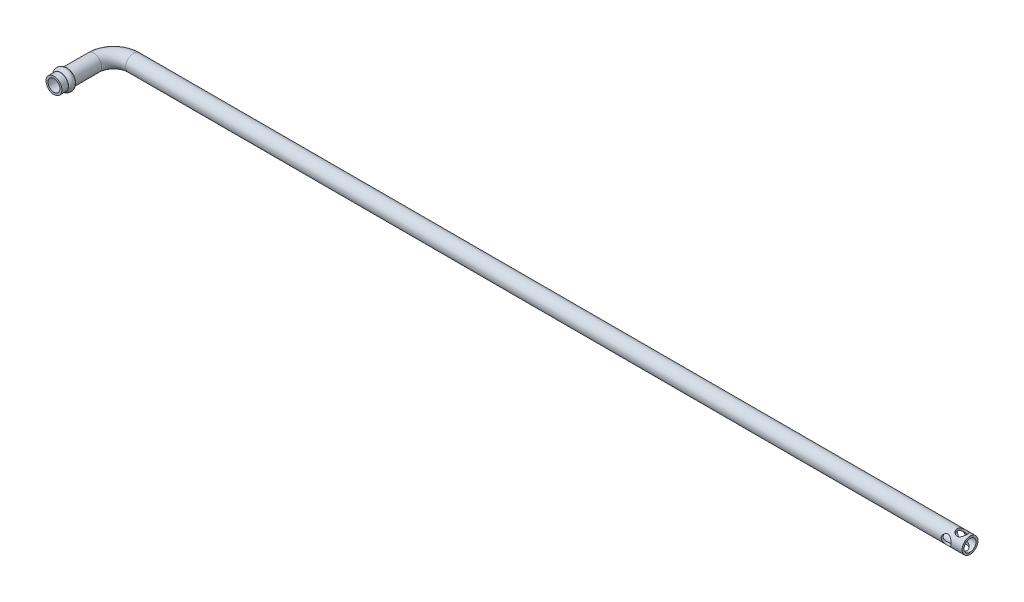
from build123d import *

# Parameters (mm, degrees)
SKETCH1_R               = 4
SKETCH1_R_2             = 3
FILLET1_R               = 0.1
CUT_EXTRUDE1_DEPTH      = 432.371069971
CUT_EXTRUDE1_DEPTH_BACK = 432.371069971
SKETCH4_R               = 2.5
CUT_EXTRUDE2_DEPTH      = 432.371070071
CUT_EXTRUDE2_DEPTH_BACK = 432.371070071
SKETCH5_R               = 2.5


with BuildPart() as part:
    # Sweep1: sweep along a path in Sketch2
    with BuildLine(Plane(origin=(0, 0, 0), x_dir=(1, 0, 0), z_dir=(0, 1, 0))) as sweep1_path:
        Line((0, 0), (0, 20))
        ThreePointArc((0, 20), (2.928932188, 27.071067812), (10, 30))
        Line((10, 30), (430, 30))
    # Sketch1 → Sweep1 (sweep)
    with BuildSketch(Plane.XY):
        Circle(SKETCH1_R)
        Circle(SKETCH1_R_2, mode=Mode.SUBTRACT)
    sweep(path=sweep1_path.line)

    # Sketch3 → Revolve1 (revolve)
    with BuildSketch(Plane(origin=(0, 0, 0), x_dir=(1, 0, 0), z_dir=(0, 1, 0)), mode=Mode.PRIVATE) as revolve1_sk:
        with BuildLine():
            Line((-4, 6.732050808), (-4, 3.267949192))
            ThreePointArc((-4, 3.267949192), (-5, 5), (-4, 6.732050808))
        make_face()
    revolve(revolve1_sk.sketch.rotate(Axis((0, 0, 0), (0, 0, -1)), 180), axis=Axis((0, 0, 0), (0, 0, -1)))

    # Fillet1
    fillet1_edges = [part.edges().sort_by_distance(p)[0] for p in [
        (-4, 0, -6.732050808),
        (-4, 0, -3.267949192),
    ]]
    fillet(fillet1_edges, radius=FILLET1_R)

    # Sketch4 → Cut-Extrude1 (cut, two sides: drawn at the far end of the back side and taken through both)
    with BuildSketch(Plane(origin=(0, 0, 0), x_dir=(1, 0, 0), z_dir=(0, 1, 0)).offset(-CUT_EXTRUDE1_DEPTH_BACK)):
        with Locations(Location((426, 30, 0), (0, 0, 270))):
            Circle(SKETCH4_R)
    extrude(amount=CUT_EXTRUDE1_DEPTH + CUT_EXTRUDE1_DEPTH_BACK, mode=Mode.SUBTRACT)

    # Sketch5 → Cut-Extrude2 (cut, two sides: drawn at the far end of the back side and taken through both)
    with BuildSketch(Plane.XY.offset(-CUT_EXTRUDE2_DEPTH_BACK)):
        with Locations((422, 0)):
            Circle(SKETCH5_R)
    extrude(amount=CUT_EXTRUDE2_DEPTH + CUT_EXTRUDE2_DEPTH_BACK, mode=Mode.SUBTRACT)


solid = part.part
